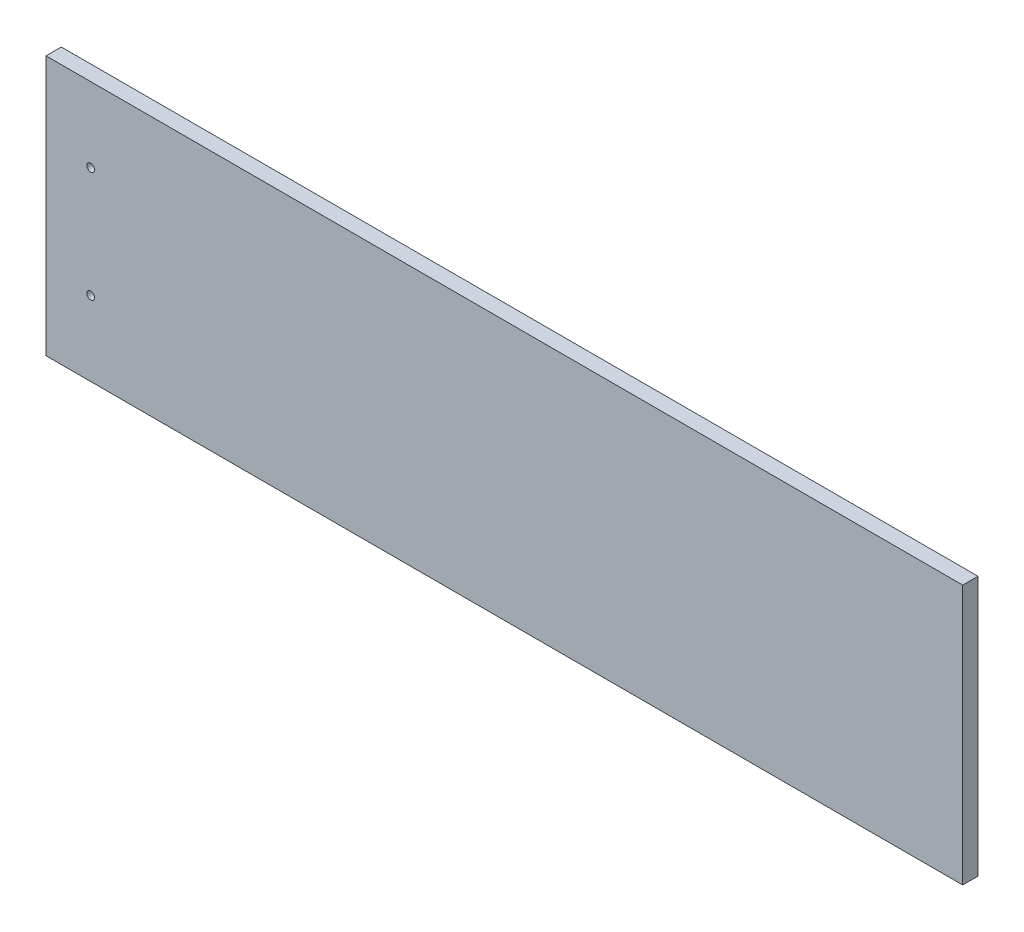
from build123d import *

# Parameters (mm, degrees)
SKETCH1_W             = 600
SKETCH1_H             = 170
BOSS_EXTRUDE1_DEPTH   = 10
M6_TAPPED_HOLE1_D     = 5
M6_TAPPED_HOLE1_DEPTH = 15
M6_TAPPED_HOLE1_TIP   = 1.502151548


with BuildPart() as part:
    # Sketch1 → Boss-Extrude1 (new body)
    with BuildSketch(Plane.XY):
        Rectangle(SKETCH1_W, SKETCH1_H)
    extrude(amount=BOSS_EXTRUDE1_DEPTH)

    # M6 Tapped Hole1
    with Locations(Plane(origin=(0, 0, 0), x_dir=(-1, 0, 0), z_dir=(0, 0, -1))):
        with Locations((270.75, 36.25), (270.75, -36.25)):
            Hole(M6_TAPPED_HOLE1_D / 2, depth=M6_TAPPED_HOLE1_DEPTH)
            with Locations((0, 0, -(M6_TAPPED_HOLE1_DEPTH + M6_TAPPED_HOLE1_TIP / 2))):  # 118° drill point
                Cone(0, M6_TAPPED_HOLE1_D / 2, M6_TAPPED_HOLE1_TIP, mode=Mode.SUBTRACT)


solid = part.part
